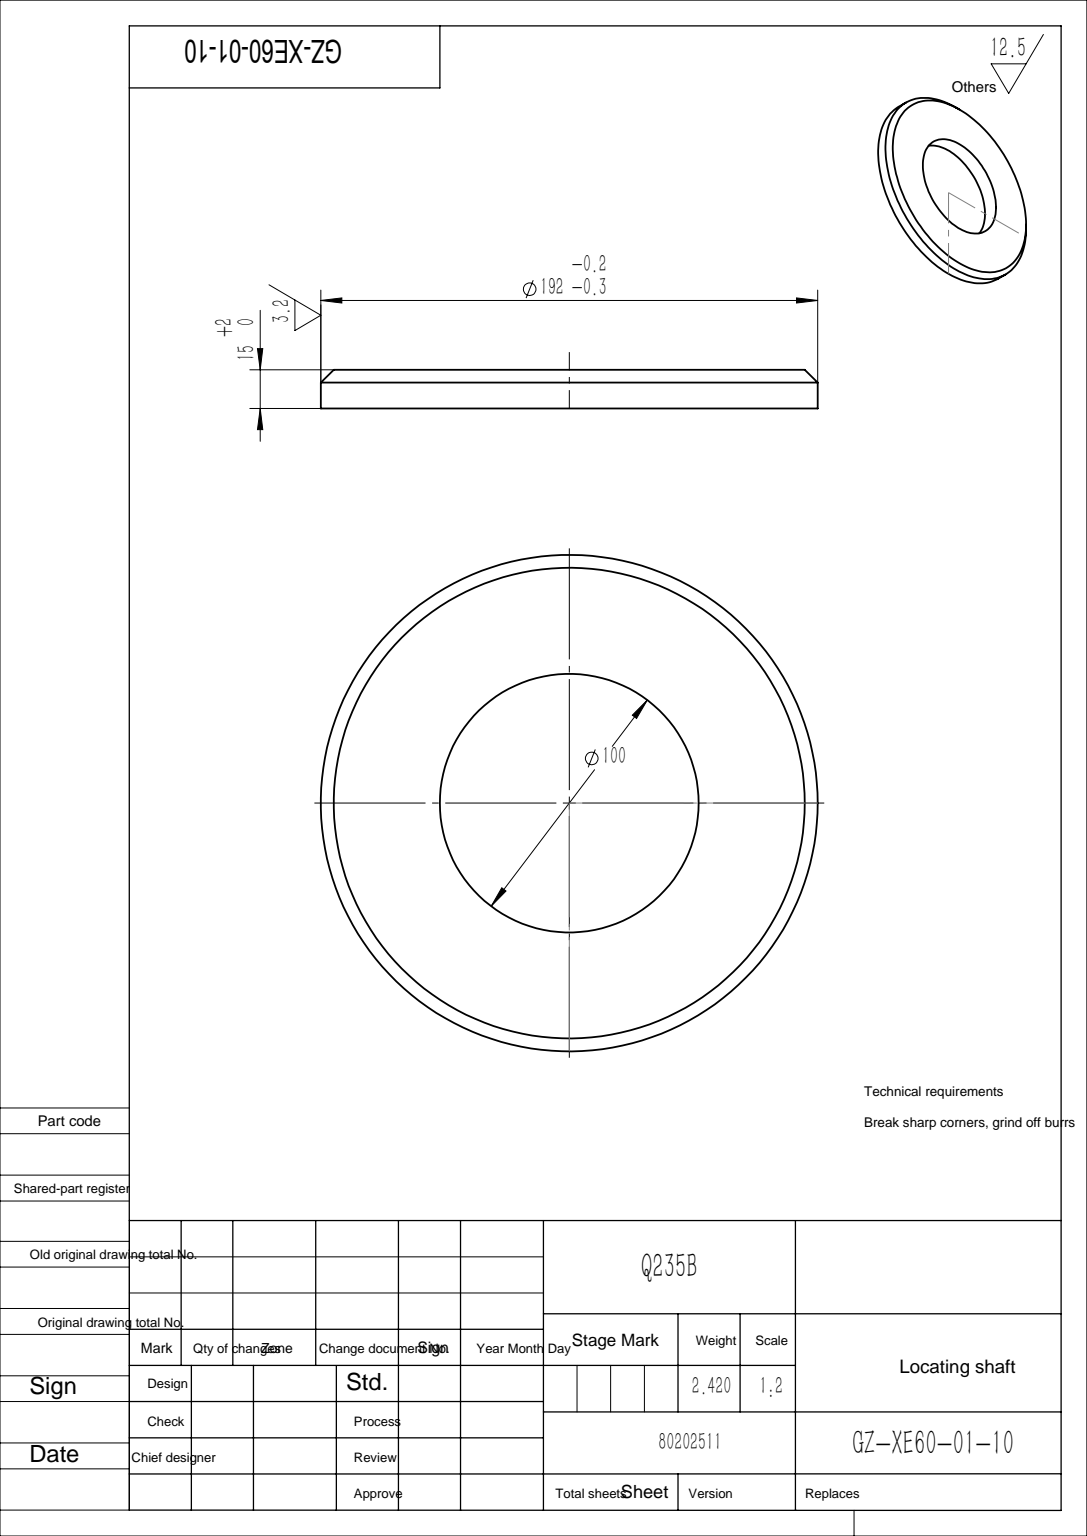
SolidWorks part; units mm, degrees
material "Q235B"
ref_plane "Front Plane" through (0, 0, 0) normal (0, 0, 1) x (1, 0, 0)
ref_plane "Top Plane" through (0, 0, 0) normal (0, 1, 0) x (1, 0, 0)
ref_plane "Right Plane" through (0, 0, 0) normal (1, 0, 0) x (0, 0, -1)
sketch "Sketch1" plane through (0, 0, 0) normal (0, 0, 1) x (1, 0, 0)
  circle A0 centre (0, 0) radius 96
  circle A1 centre (0, 0) radius 50
  dimension "D1" = 192
  dimension "D2" = 100
extrude "Boss-Extrude1" add sketch "Sketch1" along normal blind 15
sketch "Sketch2" plane through (0, 0, 0) normal (0, 0, -1) x (-1, 0, 0)
  line L0 (0, 0) -> (-96, 0) construction
  line L1 (0, 0) -> (0, -96) construction
  circle A0 centre (0, 0) radius 96 construction
chamfer "Chamfer1" distance 5 angle 45 1 edges at (96, 0, 15)
